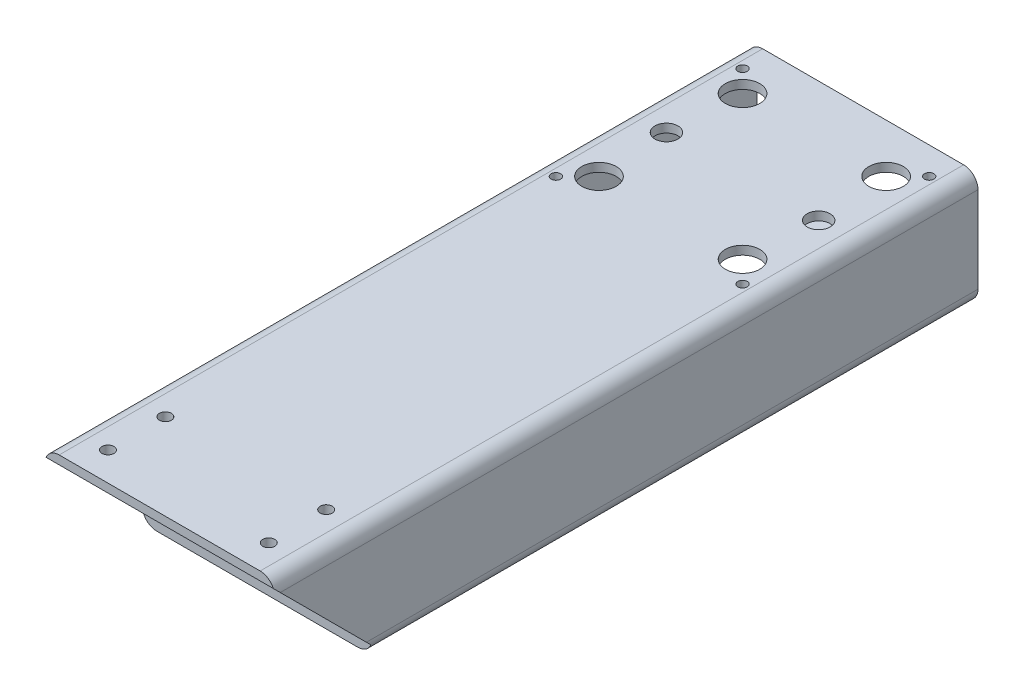
from build123d import *

# Parameters (mm, degrees)
BOSS_EXTRUDE1_DEPTH             = 245
SKETCH6_R                       = 23.25
CUT_EXTRUDE1_DEPTH              = 3
F_6_5_6_5_DIAMETER_HOLE1_D      = 6.5
F_12_0_12_DIAMETER_HOLE1_REACH  = 253.446
F_12_0_12_DIAMETER_HOLE1_BORE_R = 6
M4_TAPPED_HOLE1_REACH           = 253.446
M4_TAPPED_HOLE1_BORE_R          = 1.65
CUT_EXTRUDE2_DEPTH              = 259.505319094
SKETCH12_R                      = 5
BOSS_EXTRUDE2_DEPTH             = 3
M5_TAPPED_HOLE1_D               = 4.2
M3_TAPPED_HOLE1_D               = 2.5
M3_TAPPED_HOLE1_DEPTH           = 3
CUT_EXTRUDE3_REACH              = 253.446
SKETCH17_R                      = 4


with BuildPart() as part:
    # Sketch1 → Boss-Extrude1 (new body)
    with BuildSketch(Plane.XY):
        with BuildLine():
            Line((-35, 20), (35, 20))
            ThreePointArc((35, 20), (38.535533906, 18.535533906), (40, 15))
            Line((40, 15), (40, -15))
            ThreePointArc((40, -15), (38.535533906, -18.535533906), (35, -20))
            Line((35, -20), (-35, -20))
            ThreePointArc((-35, -20), (-38.535533906, -18.535533906), (-40, -15))
            Line((-40, -15), (-40, 15))
            ThreePointArc((-40, 15), (-38.535533906, 18.535533906), (-35, 20))
        make_face()
        with BuildLine():
            Line((-37, 15), (-37, -15))
            ThreePointArc((-37, -15), (-36.414213562, -16.414213562), (-35, -17))
            Line((-35, -17), (35, -17))
            ThreePointArc((35, -17), (36.414213562, -16.414213562), (37, -15))
            Line((37, -15), (37, 15))
            ThreePointArc((37, 15), (36.414213562, 16.414213562), (35, 17))
            Line((35, 17), (-35, 17))
            ThreePointArc((-35, 17), (-36.414213562, 16.414213562), (-37, 15))
        make_face(mode=Mode.SUBTRACT)
    extrude(amount=BOSS_EXTRUDE1_DEPTH)

    # Sketch6 → Cut-Extrude1 (cut)
    with BuildSketch(Plane.XZ.offset(20)):
        with Locations(Location((0, 42, 0), (0, 0, 270))):
            Circle(SKETCH6_R)
    extrude(amount=-CUT_EXTRUDE1_DEPTH, mode=Mode.SUBTRACT)

    # Ø6.5 (6.5) Diameter Hole1 (through all)
    with Locations(Plane(origin=(0, 20, 0), x_dir=(1, 0, 0), z_dir=(0, 1, 0))):
        with Locations((-25, -17), (25, -17), (25, -67), (-25, -67)):
            Hole(F_6_5_6_5_DIAMETER_HOLE1_D / 2)

    # Ø12.0 (12) Diameter Hole1 bore → Ø12.0 (12) Diameter Hole1 (cut, up to next)
    with BuildSketch(Plane(origin=(0, 20, 0), x_dir=(1, 0, 0), z_dir=(0, 1, 0)), mode=Mode.PRIVATE) as f_12_0_12_diameter_hole1_sk1:
        with Locations((-25, -17)):
            Circle(F_12_0_12_DIAMETER_HOLE1_BORE_R)
    f_12_0_12_diameter_hole1_tool1 = extrude(f_12_0_12_diameter_hole1_sk1.sketch, amount=-F_12_0_12_DIAMETER_HOLE1_REACH, mode=Mode.PRIVATE) & part.part
    # Ø12.0 (12) Diameter Hole1 bore → Ø12.0 (12) Diameter Hole1 (cut, up to next)
    with BuildSketch(Plane(origin=(0, 20, 0), x_dir=(1, 0, 0), z_dir=(0, 1, 0)), mode=Mode.PRIVATE) as f_12_0_12_diameter_hole1_sk2:
        with Locations((25, -17)):
            Circle(F_12_0_12_DIAMETER_HOLE1_BORE_R)
    f_12_0_12_diameter_hole1_tool2 = extrude(f_12_0_12_diameter_hole1_sk2.sketch, amount=-F_12_0_12_DIAMETER_HOLE1_REACH, mode=Mode.PRIVATE) & part.part
    # Ø12.0 (12) Diameter Hole1 bore → Ø12.0 (12) Diameter Hole1 (cut, up to next)
    with BuildSketch(Plane(origin=(0, 20, 0), x_dir=(1, 0, 0), z_dir=(0, 1, 0)), mode=Mode.PRIVATE) as f_12_0_12_diameter_hole1_sk3:
        with Locations((25, -67)):
            Circle(F_12_0_12_DIAMETER_HOLE1_BORE_R)
    f_12_0_12_diameter_hole1_tool3 = extrude(f_12_0_12_diameter_hole1_sk3.sketch, amount=-F_12_0_12_DIAMETER_HOLE1_REACH, mode=Mode.PRIVATE) & part.part
    # Ø12.0 (12) Diameter Hole1 bore → Ø12.0 (12) Diameter Hole1 (cut, up to next)
    with BuildSketch(Plane(origin=(0, 20, 0), x_dir=(1, 0, 0), z_dir=(0, 1, 0)), mode=Mode.PRIVATE) as f_12_0_12_diameter_hole1_sk4:
        with Locations((-25, -67)):
            Circle(F_12_0_12_DIAMETER_HOLE1_BORE_R)
    f_12_0_12_diameter_hole1_tool4 = extrude(f_12_0_12_diameter_hole1_sk4.sketch, amount=-F_12_0_12_DIAMETER_HOLE1_REACH, mode=Mode.PRIVATE) & part.part
    add(f_12_0_12_diameter_hole1_tool1.solids().sort_by_distance((-25, 20, 17))[0], mode=Mode.SUBTRACT)
    add(f_12_0_12_diameter_hole1_tool2.solids().sort_by_distance((25, 20, 17))[0], mode=Mode.SUBTRACT)
    add(f_12_0_12_diameter_hole1_tool3.solids().sort_by_distance((25, 20, 67))[0], mode=Mode.SUBTRACT)
    add(f_12_0_12_diameter_hole1_tool4.solids().sort_by_distance((-25, 20, 67))[0], mode=Mode.SUBTRACT)

    # M4 Tapped Hole1 bore → M4 Tapped Hole1 (cut, up to next)
    with BuildSketch(Plane(origin=(0, 20, 0), x_dir=(1, 0, 0), z_dir=(0, 1, 0)), mode=Mode.PRIVATE) as m4_tapped_hole1_sk1:
        with Locations((-32.5, -9.5)):
            Circle(M4_TAPPED_HOLE1_BORE_R)
    m4_tapped_hole1_tool1 = extrude(m4_tapped_hole1_sk1.sketch, amount=-M4_TAPPED_HOLE1_REACH, mode=Mode.PRIVATE) & part.part
    # M4 Tapped Hole1 bore → M4 Tapped Hole1 (cut, up to next)
    with BuildSketch(Plane(origin=(0, 20, 0), x_dir=(1, 0, 0), z_dir=(0, 1, 0)), mode=Mode.PRIVATE) as m4_tapped_hole1_sk2:
        with Locations((32.5, -9.5)):
            Circle(M4_TAPPED_HOLE1_BORE_R)
    m4_tapped_hole1_tool2 = extrude(m4_tapped_hole1_sk2.sketch, amount=-M4_TAPPED_HOLE1_REACH, mode=Mode.PRIVATE) & part.part
    # M4 Tapped Hole1 bore → M4 Tapped Hole1 (cut, up to next)
    with BuildSketch(Plane(origin=(0, 20, 0), x_dir=(1, 0, 0), z_dir=(0, 1, 0)), mode=Mode.PRIVATE) as m4_tapped_hole1_sk3:
        with Locations((32.5, -74.5)):
            Circle(M4_TAPPED_HOLE1_BORE_R)
    m4_tapped_hole1_tool3 = extrude(m4_tapped_hole1_sk3.sketch, amount=-M4_TAPPED_HOLE1_REACH, mode=Mode.PRIVATE) & part.part
    # M4 Tapped Hole1 bore → M4 Tapped Hole1 (cut, up to next)
    with BuildSketch(Plane(origin=(0, 20, 0), x_dir=(1, 0, 0), z_dir=(0, 1, 0)), mode=Mode.PRIVATE) as m4_tapped_hole1_sk4:
        with Locations((-32.5, -74.5)):
            Circle(M4_TAPPED_HOLE1_BORE_R)
    m4_tapped_hole1_tool4 = extrude(m4_tapped_hole1_sk4.sketch, amount=-M4_TAPPED_HOLE1_REACH, mode=Mode.PRIVATE) & part.part
    add(m4_tapped_hole1_tool1.solids().sort_by_distance((-32.5, 20, 9.5))[0], mode=Mode.SUBTRACT)
    add(m4_tapped_hole1_tool2.solids().sort_by_distance((32.5, 20, 9.5))[0], mode=Mode.SUBTRACT)
    add(m4_tapped_hole1_tool3.solids().sort_by_distance((32.5, 20, 74.5))[0], mode=Mode.SUBTRACT)
    add(m4_tapped_hole1_tool4.solids().sort_by_distance((-32.5, 20, 74.5))[0], mode=Mode.SUBTRACT)

    # Sketch9 → Cut-Extrude2 (cut, through all)
    with BuildSketch(Plane(origin=(40, 0, 0), x_dir=(0, 0, -1), z_dir=(1, 0, 0))):
        Polygon((-245, 17), (-245, -20), (-211, -20), (-211, -17), align=None)
    extrude(amount=-CUT_EXTRUDE2_DEPTH, mode=Mode.SUBTRACT)

    # Sketch12 → Boss-Extrude2 (add)
    with BuildSketch(Plane.XZ.offset(-17)):
        with Locations((-28, 215)):
            Circle(SKETCH12_R)
        with Locations((-28, 235)):
            Circle(SKETCH12_R)
        with Locations((28, 215)):
            Circle(SKETCH12_R)
        with Locations((28, 235)):
            Circle(SKETCH12_R)
    extrude(amount=BOSS_EXTRUDE2_DEPTH)

    # M5 Tapped Hole1 (through all)
    with Locations(Plane(origin=(-35, 20, 20), x_dir=(1, 0, 0), z_dir=(0, 1, 0))):
        with Locations((7, -195), (7, -215), (63, -195), (63, -215)):
            Hole(M5_TAPPED_HOLE1_D / 2)

    # M3 Tapped Hole1
    with Locations(Plane(origin=(0, -20, 0), x_dir=(-1, 0, 0), z_dir=(0, -1, 0))):
        with Locations((26.5, -42), (-26.5, -42)):
            Hole(M3_TAPPED_HOLE1_D / 2, depth=M3_TAPPED_HOLE1_DEPTH)

    # Sketch17 → Cut-Extrude3 (cut, up to next)
    with BuildSketch(Plane(origin=(0, 20, 0), x_dir=(1, 0, 0), z_dir=(0, 1, 0)), mode=Mode.PRIVATE) as cut_extrude3_sk1:
        with Locations(Location((-26.5, -42, 0), (0, 0, 270))):
            Circle(SKETCH17_R)
    cut_extrude3_tool1 = extrude(cut_extrude3_sk1.sketch, amount=-CUT_EXTRUDE3_REACH, mode=Mode.PRIVATE) & part.part
    # Sketch17 → Cut-Extrude3 (cut, up to next)
    with BuildSketch(Plane(origin=(0, 20, 0), x_dir=(1, 0, 0), z_dir=(0, 1, 0)), mode=Mode.PRIVATE) as cut_extrude3_sk2:
        with Locations(Location((26.5, -42, 0), (0, 0, 270))):
            Circle(SKETCH17_R)
    cut_extrude3_tool2 = extrude(cut_extrude3_sk2.sketch, amount=-CUT_EXTRUDE3_REACH, mode=Mode.PRIVATE) & part.part
    add(cut_extrude3_tool1.solids().sort_by_distance((-26.5, 20, 42))[0], mode=Mode.SUBTRACT)
    add(cut_extrude3_tool2.solids().sort_by_distance((26.5, 20, 42))[0], mode=Mode.SUBTRACT)


solid = part.part
